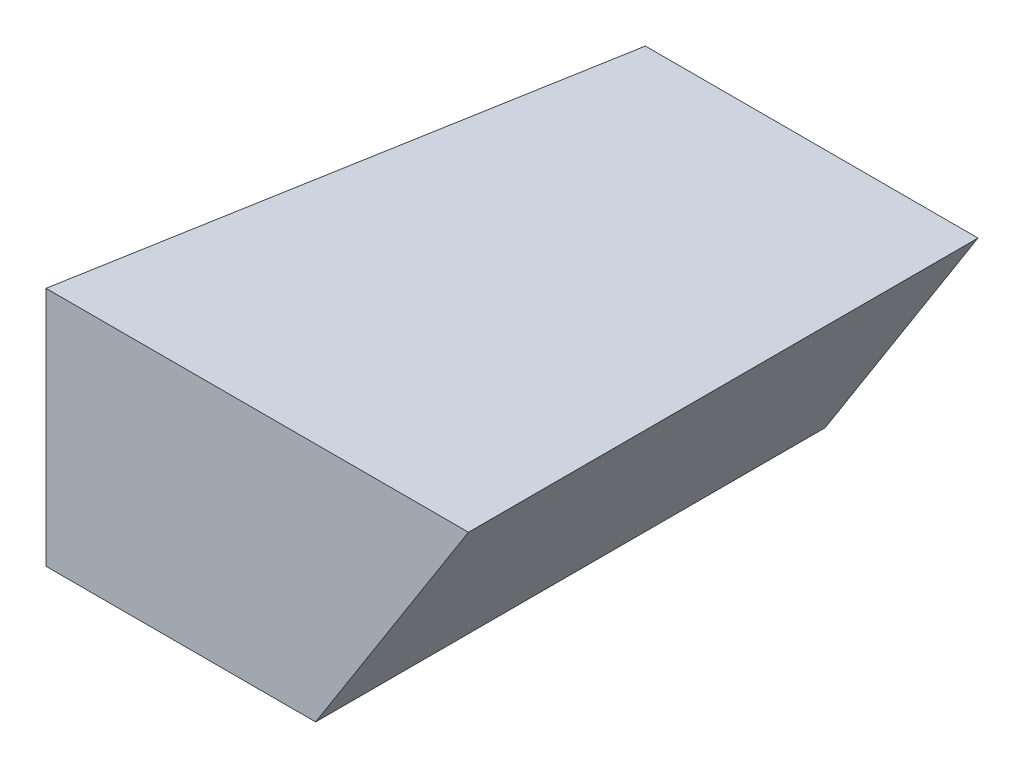
from build123d import *

# Parameters (mm, degrees)
EXTRUDE_1_DEPTH     = 3.175
CUT_EXTRUDE_1_DEPTH = 10


with BuildPart() as part:
    # 草图1 → 凸台-拉伸1 (new body)
    with BuildSketch(Plane.XY):
        Polygon((-4.407915319, 5), (-7.407915319, 5), (-7.407915319, 6.5), (-3.455415319, 6.5), align=None)
    extrude(amount=EXTRUDE_1_DEPTH)

    # 草图2 → 切除-拉伸1 (cut)
    with BuildSketch(Plane.XZ.offset(-5)):
        Polygon((-7.407915319, 0), (-5.527915319, 0), (-6.087915319, 3.175), (-7.407915319, 3.175), align=None)
    extrude(amount=-CUT_EXTRUDE_1_DEPTH, mode=Mode.SUBTRACT)


solid = part.part
